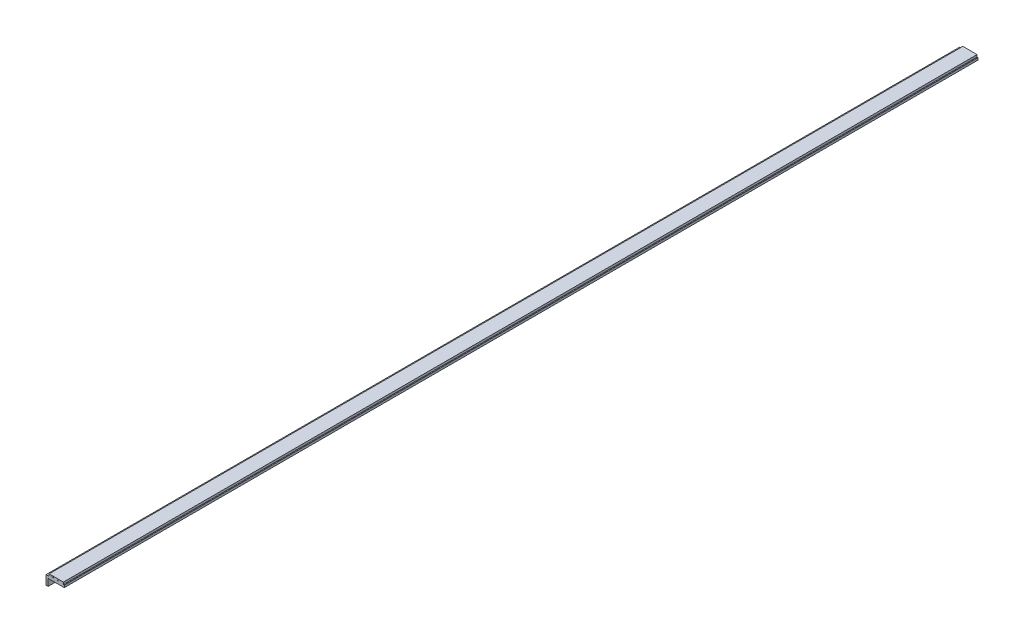
from build123d import *

# Parameters (mm, degrees)
BOSS_EXTRUDE1_DEPTH      = 5000
SKETCH2_W                = 1.259860676
SKETCH2_H                = 9.043092937
CUT_EXTRUDE1_DEPTH       = 0.2
LPATTERN1_COUNT          = 16
LPATTERN1_PITCH          = 6
MIRROR1_COPY_1_SKETCH_W  = 1.259860676
MIRROR1_COPY_1_SKETCH_H  = 9.043092937
MIRROR1_COPY_1_DEPTH     = 0.2
MIRROR1_COPY_2_SKETCH_W  = 1.259860676
MIRROR1_COPY_2_SKETCH_H  = 9.043092937
MIRROR1_COPY_2_DEPTH     = 0.2
MIRROR1_COPY_3_SKETCH_W  = 1.259860676
MIRROR1_COPY_3_SKETCH_H  = 9.043092937
MIRROR1_COPY_3_DEPTH     = 0.2
MIRROR1_COPY_4_SKETCH_W  = 1.259860676
MIRROR1_COPY_4_SKETCH_H  = 9.043092937
MIRROR1_COPY_4_DEPTH     = 0.2
MIRROR1_COPY_5_SKETCH_W  = 1.259860676
MIRROR1_COPY_5_SKETCH_H  = 9.043092937
MIRROR1_COPY_5_DEPTH     = 0.2
MIRROR1_COPY_6_SKETCH_W  = 1.259860676
MIRROR1_COPY_6_SKETCH_H  = 9.043092937
MIRROR1_COPY_6_DEPTH     = 0.2
MIRROR1_COPY_7_SKETCH_W  = 1.259860676
MIRROR1_COPY_7_SKETCH_H  = 9.043092937
MIRROR1_COPY_7_DEPTH     = 0.2
MIRROR1_COPY_8_SKETCH_W  = 1.259860676
MIRROR1_COPY_8_SKETCH_H  = 9.043092937
MIRROR1_COPY_8_DEPTH     = 0.2
MIRROR1_COPY_9_SKETCH_W  = 1.259860676
MIRROR1_COPY_9_SKETCH_H  = 9.043092937
MIRROR1_COPY_9_DEPTH     = 0.2
MIRROR1_COPY_10_SKETCH_W = 1.259860676
MIRROR1_COPY_10_SKETCH_H = 9.043092937
MIRROR1_COPY_10_DEPTH    = 0.2
MIRROR1_COPY_11_SKETCH_W = 1.259860676
MIRROR1_COPY_11_SKETCH_H = 9.043092937
MIRROR1_COPY_11_DEPTH    = 0.2
MIRROR1_COPY_12_SKETCH_W = 1.259860676
MIRROR1_COPY_12_SKETCH_H = 9.043092937
MIRROR1_COPY_12_DEPTH    = 0.2
MIRROR1_COPY_13_SKETCH_W = 1.259860676
MIRROR1_COPY_13_SKETCH_H = 9.043092937
MIRROR1_COPY_13_DEPTH    = 0.2
MIRROR1_COPY_14_SKETCH_W = 1.259860676
MIRROR1_COPY_14_SKETCH_H = 9.043092937
MIRROR1_COPY_14_DEPTH    = 0.2
MIRROR1_COPY_15_SKETCH_W = 1.259860676
MIRROR1_COPY_15_SKETCH_H = 9.043092937
MIRROR1_COPY_15_DEPTH    = 0.2
SKETCH3_W                = 12
SKETCH3_H                = 50
BOSS_EXTRUDE2_DEPTH      = 5000
SKETCH4_W                = 12
SKETCH4_H                = 88
CUT_EXTRUDE2_DEPTH       = 5002.99960016


with BuildPart() as part:
    # Sketch1 → Boss-Extrude1 (new body)
    with BuildSketch(Plane.XY):
        Polygon((0, 0), (100, 0), (100, 12), (95, 12), (95, 24), (17, 24), (17, 12), (12, 12), (12, 100), (0, 100), align=None)
    extrude(amount=BOSS_EXTRUDE1_DEPTH)

    # Sketch2 → Cut-Extrude1 (cut)
    with BuildSketch(Plane.XY.offset(5000)):
        with Locations((22.109179897, 19.478453532)):
            Rectangle(SKETCH2_W, SKETCH2_H)
    cut_extrude1 = extrude(amount=-CUT_EXTRUDE1_DEPTH, mode=Mode.SUBTRACT)

    # LPattern1: Cut-Extrude1 ×16
    with Locations(*[(i * LPATTERN1_PITCH, 0, 0) for i in range(1, LPATTERN1_COUNT)]):
        add(cut_extrude1, mode=Mode.SUBTRACT)

    # Mirror1: Cut-Extrude1 across plane
    add(cut_extrude1.mirror(Plane(origin=(0, 0, 2500), x_dir=(1, 0, 0), z_dir=(0, 0, -1))), mode=Mode.SUBTRACT)

    # Mirror1 copy 1 sketch → Mirror1 copy 1 (cut)
    with BuildSketch(Plane(origin=(6, 0, 0), x_dir=(1, 0, 0), z_dir=(0, 0, -1))):
        with Locations((22.109179897, -19.478453532)):
            Rectangle(MIRROR1_COPY_1_SKETCH_W, MIRROR1_COPY_1_SKETCH_H)
    extrude(amount=-MIRROR1_COPY_1_DEPTH, mode=Mode.SUBTRACT)

    # Mirror1 copy 2 sketch → Mirror1 copy 2 (cut)
    with BuildSketch(Plane(origin=(12, 0, 0), x_dir=(1, 0, 0), z_dir=(0, 0, -1))):
        with Locations((22.109179897, -19.478453532)):
            Rectangle(MIRROR1_COPY_2_SKETCH_W, MIRROR1_COPY_2_SKETCH_H)
    extrude(amount=-MIRROR1_COPY_2_DEPTH, mode=Mode.SUBTRACT)

    # Mirror1 copy 3 sketch → Mirror1 copy 3 (cut)
    with BuildSketch(Plane(origin=(18, 0, 0), x_dir=(1, 0, 0), z_dir=(0, 0, -1))):
        with Locations((22.109179897, -19.478453532)):
            Rectangle(MIRROR1_COPY_3_SKETCH_W, MIRROR1_COPY_3_SKETCH_H)
    extrude(amount=-MIRROR1_COPY_3_DEPTH, mode=Mode.SUBTRACT)

    # Mirror1 copy 4 sketch → Mirror1 copy 4 (cut)
    with BuildSketch(Plane(origin=(24, 0, 0), x_dir=(1, 0, 0), z_dir=(0, 0, -1))):
        with Locations((22.109179897, -19.478453532)):
            Rectangle(MIRROR1_COPY_4_SKETCH_W, MIRROR1_COPY_4_SKETCH_H)
    extrude(amount=-MIRROR1_COPY_4_DEPTH, mode=Mode.SUBTRACT)

    # Mirror1 copy 5 sketch → Mirror1 copy 5 (cut)
    with BuildSketch(Plane(origin=(30, 0, 0), x_dir=(1, 0, 0), z_dir=(0, 0, -1))):
        with Locations((22.109179897, -19.478453532)):
            Rectangle(MIRROR1_COPY_5_SKETCH_W, MIRROR1_COPY_5_SKETCH_H)
    extrude(amount=-MIRROR1_COPY_5_DEPTH, mode=Mode.SUBTRACT)

    # Mirror1 copy 6 sketch → Mirror1 copy 6 (cut)
    with BuildSketch(Plane(origin=(36, 0, 0), x_dir=(1, 0, 0), z_dir=(0, 0, -1))):
        with Locations((22.109179897, -19.478453532)):
            Rectangle(MIRROR1_COPY_6_SKETCH_W, MIRROR1_COPY_6_SKETCH_H)
    extrude(amount=-MIRROR1_COPY_6_DEPTH, mode=Mode.SUBTRACT)

    # Mirror1 copy 7 sketch → Mirror1 copy 7 (cut)
    with BuildSketch(Plane(origin=(42, 0, 0), x_dir=(1, 0, 0), z_dir=(0, 0, -1))):
        with Locations((22.109179897, -19.478453532)):
            Rectangle(MIRROR1_COPY_7_SKETCH_W, MIRROR1_COPY_7_SKETCH_H)
    extrude(amount=-MIRROR1_COPY_7_DEPTH, mode=Mode.SUBTRACT)

    # Mirror1 copy 8 sketch → Mirror1 copy 8 (cut)
    with BuildSketch(Plane(origin=(48, 0, 0), x_dir=(1, 0, 0), z_dir=(0, 0, -1))):
        with Locations((22.109179897, -19.478453532)):
            Rectangle(MIRROR1_COPY_8_SKETCH_W, MIRROR1_COPY_8_SKETCH_H)
    extrude(amount=-MIRROR1_COPY_8_DEPTH, mode=Mode.SUBTRACT)

    # Mirror1 copy 9 sketch → Mirror1 copy 9 (cut)
    with BuildSketch(Plane(origin=(54, 0, 0), x_dir=(1, 0, 0), z_dir=(0, 0, -1))):
        with Locations((22.109179897, -19.478453532)):
            Rectangle(MIRROR1_COPY_9_SKETCH_W, MIRROR1_COPY_9_SKETCH_H)
    extrude(amount=-MIRROR1_COPY_9_DEPTH, mode=Mode.SUBTRACT)

    # Mirror1 copy 10 sketch → Mirror1 copy 10 (cut)
    with BuildSketch(Plane(origin=(60, 0, 0), x_dir=(1, 0, 0), z_dir=(0, 0, -1))):
        with Locations((22.109179897, -19.478453532)):
            Rectangle(MIRROR1_COPY_10_SKETCH_W, MIRROR1_COPY_10_SKETCH_H)
    extrude(amount=-MIRROR1_COPY_10_DEPTH, mode=Mode.SUBTRACT)

    # Mirror1 copy 11 sketch → Mirror1 copy 11 (cut)
    with BuildSketch(Plane(origin=(66, 0, 0), x_dir=(1, 0, 0), z_dir=(0, 0, -1))):
        with Locations((22.109179897, -19.478453532)):
            Rectangle(MIRROR1_COPY_11_SKETCH_W, MIRROR1_COPY_11_SKETCH_H)
    extrude(amount=-MIRROR1_COPY_11_DEPTH, mode=Mode.SUBTRACT)

    # Mirror1 copy 12 sketch → Mirror1 copy 12 (cut)
    with BuildSketch(Plane(origin=(72, 0, 0), x_dir=(1, 0, 0), z_dir=(0, 0, -1))):
        with Locations((22.109179897, -19.478453532)):
            Rectangle(MIRROR1_COPY_12_SKETCH_W, MIRROR1_COPY_12_SKETCH_H)
    extrude(amount=-MIRROR1_COPY_12_DEPTH, mode=Mode.SUBTRACT)

    # Mirror1 copy 13 sketch → Mirror1 copy 13 (cut)
    with BuildSketch(Plane(origin=(78, 0, 0), x_dir=(1, 0, 0), z_dir=(0, 0, -1))):
        with Locations((22.109179897, -19.478453532)):
            Rectangle(MIRROR1_COPY_13_SKETCH_W, MIRROR1_COPY_13_SKETCH_H)
    extrude(amount=-MIRROR1_COPY_13_DEPTH, mode=Mode.SUBTRACT)

    # Mirror1 copy 14 sketch → Mirror1 copy 14 (cut)
    with BuildSketch(Plane(origin=(84, 0, 0), x_dir=(1, 0, 0), z_dir=(0, 0, -1))):
        with Locations((22.109179897, -19.478453532)):
            Rectangle(MIRROR1_COPY_14_SKETCH_W, MIRROR1_COPY_14_SKETCH_H)
    extrude(amount=-MIRROR1_COPY_14_DEPTH, mode=Mode.SUBTRACT)

    # Mirror1 copy 15 sketch → Mirror1 copy 15 (cut)
    with BuildSketch(Plane(origin=(90, 0, 0), x_dir=(1, 0, 0), z_dir=(0, 0, -1))):
        with Locations((22.109179897, -19.478453532)):
            Rectangle(MIRROR1_COPY_15_SKETCH_W, MIRROR1_COPY_15_SKETCH_H)
    extrude(amount=-MIRROR1_COPY_15_DEPTH, mode=Mode.SUBTRACT)

    # Sketch3 → Boss-Extrude2 (add)
    with BuildSketch(Plane.XY.offset(5000)):
        with Locations((6, -13)):
            Rectangle(SKETCH3_W, SKETCH3_H)
    extrude(amount=-BOSS_EXTRUDE2_DEPTH)

    # Sketch4 → Cut-Extrude2 (cut, through all)
    with BuildSketch(Plane(origin=(0, 0, 0), x_dir=(-1, 0, 0), z_dir=(0, 0, -1))):
        with Locations((-6, 56)):
            Rectangle(SKETCH4_W, SKETCH4_H)
    extrude(amount=-CUT_EXTRUDE2_DEPTH, mode=Mode.SUBTRACT)


solid = part.part
